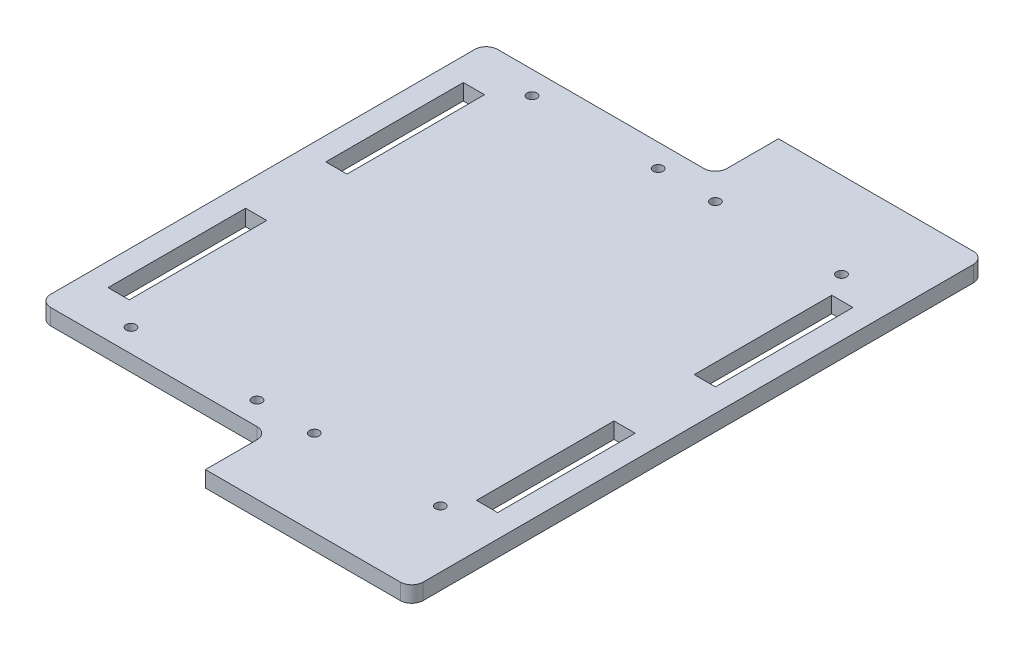
SolidWorks part; units mm, degrees
material "Q235"
ref_plane "Front Plane" through (0, 0, 0) normal (0, 0, 1) x (1, 0, 0)
ref_plane "Top Plane" through (0, 0, 0) normal (0, 1, 0) x (1, 0, 0)
ref_plane "Right Plane" through (0, 0, 0) normal (1, 0, 0) x (0, 0, -1)
sketch "Sketch1" plane through (0, 0, 0) normal (0, 1, 0) x (1, 0, 0)
  line L1 (-190, 250) -> (190, 250)
  line L2 (-190, 250) -> (-190, -250)
  line L3 (-190, -250) -> (190, -250)
  line L4 (190, 250) -> (190, -250)
  line L5 (-190, 250) -> (190, -250) construction
  line L6 (-190, -250) -> (190, 250) construction
  point P0 (0, 0)
  dimension "D1" = 380
  dimension "D2" = 500
extrude "Boss-Extrude1" add sketch "Sketch1" along normal blind 14
sketch "Sketch2" plane through (0, 14, 0) normal (0, 1, 0) x (1, 0, 0)
  line L0 (-190, 0) -> (-39.9367, 0) construction
  line L1 (-190, 250) -> (10, 250)
  line L2 (-190, 250) -> (-190, 195)
  line L3 (-190, 195) -> (10, 195)
  line L4 (10, 250) -> (10, 195)
  line L5 (-190, 250) -> (-190, -250) construction
  line L6 (10, -250) -> (10, -195)
  line L7 (-190, -195) -> (10, -195)
  line L8 (-190, -250) -> (-190, -195)
  line L9 (-190, -250) -> (10, -250)
  dimension "D1" = 390
  dimension "D2" = 200
extrude "Cut-Extrude1" cut sketch "Sketch2" against normal blind 14
fillet "Fillet1" radius 10 2 edges at (10, 7, -195) (10, 7, 195)
sketch "Sketch3" plane through (0, 14, 0) normal (0, 1, 0) x (1, 0, 0)
  line L0 (190, 0) -> (151.2269, 0) construction
  line L1 (151.5, 155) -> (170, 155)
  line L2 (151.5, 155) -> (151.5, 35)
  line L3 (151.5, 35) -> (170, 35)
  line L4 (170, 155) -> (170, 35)
  line L5 (190, -250) -> (190, 250) construction
  line L6 (170, -155) -> (170, -35)
  line L7 (151.5, -35) -> (170, -35)
  line L8 (151.5, -155) -> (151.5, -35)
  line L9 (151.5, -155) -> (170, -155)
  line L10 (0, 0) -> (0, 91.9581) construction
  line L11 (-151.5, -155) -> (-170, -155)
  line L12 (-151.5, -155) -> (-151.5, -35)
  line L13 (-151.5, -35) -> (-170, -35)
  line L14 (-170, -155) -> (-170, -35)
  line L15 (-170, 155) -> (-170, 35)
  line L16 (-151.5, 35) -> (-170, 35)
  line L17 (-151.5, 155) -> (-151.5, 35)
  line L18 (-151.5, 155) -> (-170, 155)
  dimension "D1" = 20
  dimension "D2" = 70
  dimension "D3" = 120
  dimension "D4" = 18.5
extrude "Cut-Extrude2" cut sketch "Sketch3" against normal blind 20
hole_wizard "M10 Tapped Hole1" positions "Sketch4" profile "Sketch5" tap size "M10" standard "GB"
sketch "Sketch4" plane through (0, 14, 0) normal (0, 1, 0) x (1, 0, 0)
  line L0 (-190, 0) -> (-185.8558, 0) construction
  line L1 (-190, 195) -> (-190, -195) construction
  line L3 (190, -250) -> (190, 250) construction
  point P0 (30, -175)
  point P2 (140, -175)
  point P11 (140, 175)
  point P12 (30, 175)
  dimension "D1" = 110
  dimension "D2" = 50
  dimension "D3" = 350
sketch "Sketch5" plane through (30, 14, 175) normal (1, 0, 0) x (0, 0, 1)
  line L0 (0, 0) -> (0, 55.5537)
  line L1 (0, 55.5537) -> (4.25, 53)
  line L2 (4.25, 53) -> (4.25, 0)
  line L5 (4.25, 0) -> (0, 0)
  line L10 (0, 55.5537) -> (-4.25, 53) construction
  line L11 (0, -6.35) -> (0, 107.95) construction
  dimension "螺纹孔钻头直径" = 8.5
  dimension "螺纹孔钻头深度" = 53
  dimension "导头角度" = 118
cosmetic thread "Cosmetic thread1" parameters "D1"=12, "D2"=10
cosmetic thread "Cosmetic thread2" parameters "D1"=12, "D2"=10
cosmetic thread "Cosmetic thread3" parameters "D1"=12, "D2"=10
cosmetic thread "Cosmetic thread4" parameters "D1"=12, "D2"=10
pattern_linear "LPattern1" count 2 spacing 160 along (-1, 0, 0) of "M10 Tapped Hole1"
fillet "Fillet2" radius 10 4 edges at (190, 7, 250) (-190, 7, 195) (-190, 7, -195) (190, 7, -250)
